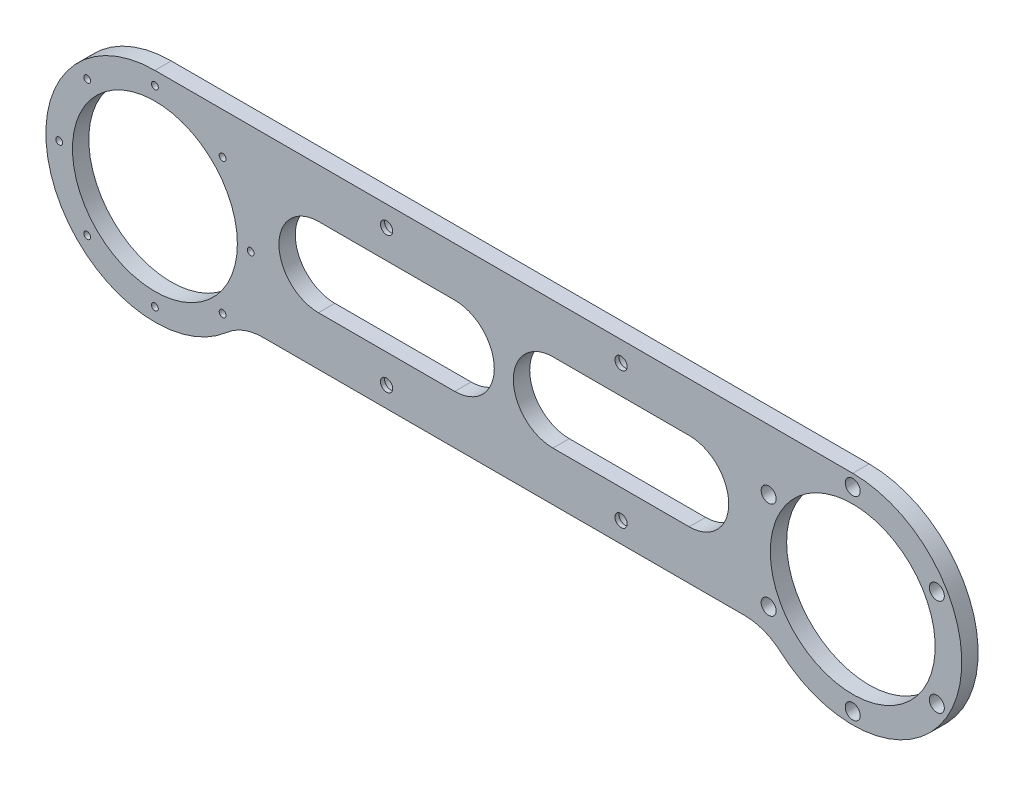
from build123d import *

# Parameters (mm, degrees)
SKETCH_1_R                   = 60.5
EXTRUDE_2_DEPTH              = 12
SKETCH_3_R                   = 60.5
CUT_EXTRUDE_2_DEPTH          = 4
HOLE_WIZARD_M8_2_D           = 9
HOLE_WIZARD_M8_2_CBORE_D     = 15
HOLE_WIZARD_M8_2_CBORE_DEPTH = 9
SKETCH_11_R                  = 18
CUT_EXTRUDE_5_DEPTH          = 472.497806181
SKETCH_12_R                  = 2.5
CUT_EXTRUDE_6_DEPTH          = 472.497806181
SKETCH_13_R                  = 60.5
CUT_EXTRUDE_7_DEPTH          = 472.412962521
SKETCH_14_R                  = 5.5
CUT_EXTRUDE_8_DEPTH          = 472.497806181


with BuildPart() as part:
    # 草图1 → 凸台-拉伸2 (new body)
    with BuildSketch(Plane.XY):
        with BuildLine():
            Line((-128, 82.886556409), (384, 82.886556409))
            ThreePointArc((384, 82.886556409), (458.833147735, -25.397714839), (331.084973779, -57.113443591))
            ThreePointArc((331.084973779, -57.113443591), (318.769596292, -49.696869724), (304.627460668, -47.113443591))
            Line((304.627460668, -47.113443591), (-48.627460668, -47.113443591))
            ThreePointArc((-48.627460668, -47.113443591), (-62.769596292, -49.696869724), (-75.084973779, -57.113443591))
            ThreePointArc((-75.084973779, -57.113443591), (-202.833147735, -25.397714839), (-128, 82.886556409))
        make_face()
        with Locations((-128, 2.886556409)):
            Circle(SKETCH_1_R, mode=Mode.SUBTRACT)
        with BuildLine():
            Line((-8, 46.886556409), (92, 46.886556409))
            ThreePointArc((92, 46.886556409), (121, 17.886556409), (92, -11.113443591))
            Line((92, -11.113443591), (-8, -11.113443591))
            ThreePointArc((-8, -11.113443591), (-37, 17.886556409), (-8, 46.886556409))
        make_face(mode=Mode.SUBTRACT)
        with BuildLine():
            Line((164, 46.886556409), (264, 46.886556409))
            ThreePointArc((264, 46.886556409), (293, 17.886556409), (264, -11.113443591))
            Line((264, -11.113443591), (164, -11.113443591))
            ThreePointArc((164, -11.113443591), (135, 17.886556409), (164, 46.886556409))
        make_face(mode=Mode.SUBTRACT)
    extrude(amount=EXTRUDE_2_DEPTH)

    # 草图3 → 切除-拉伸2 (cut)
    with BuildSketch(Plane.XY):
        with Locations((384, 2.886556409)):
            Circle(SKETCH_3_R)
    extrude(amount=CUT_EXTRUDE_2_DEPTH, mode=Mode.SUBTRACT)

    # M8 六角圆柱头螺钉的柱形沉头孔2 (through all)
    with Locations(Plane(origin=(0, 0, 0), x_dir=(-1, 0, 0), z_dir=(0, 0, -1))):
        with Locations((-214, 67.886556409), (-214, -32.113443591), (-42, 67.886556409), (-42, -32.113443591)):
            CounterBoreHole(HOLE_WIZARD_M8_2_D / 2, HOLE_WIZARD_M8_2_CBORE_D / 2, HOLE_WIZARD_M8_2_CBORE_DEPTH)

    # 草图11 → 切除-拉伸5 (cut, through all)
    with BuildSketch(Plane.XY):
        with Locations((384, 2.886556409)):
            Circle(SKETCH_11_R)
    extrude(amount=CUT_EXTRUDE_5_DEPTH, mode=Mode.SUBTRACT)

    # 草图12 → 切除-拉伸6 (cut, through all)
    with BuildSketch(Plane.XY.offset(12)):
        with Locations((-78.325748622, 52.560807787)):
            Circle(SKETCH_12_R)
        with Locations((-128, 73.136556409)):
            Circle(SKETCH_12_R)
        with Locations((-57.75, 2.886556409)):
            Circle(SKETCH_12_R)
        with Locations((-78.325748622, -46.78769497)):
            Circle(SKETCH_12_R)
        with Locations((-128, -67.363443591)):
            Circle(SKETCH_12_R)
        with Locations((-177.674251378, -46.78769497)):
            Circle(SKETCH_12_R)
        with Locations((-198.25, 2.886556409)):
            Circle(SKETCH_12_R)
        with Locations((-177.674251378, 52.560807787)):
            Circle(SKETCH_12_R)
    extrude(amount=-CUT_EXTRUDE_6_DEPTH, mode=Mode.SUBTRACT)

    # 草图13 → 切除-拉伸7 (cut, through all)
    with BuildSketch(Plane(origin=(0, 0, 4), x_dir=(-1, 0, 0), z_dir=(0, 0, -1))):
        with Locations((-384, 2.886556409)):
            Circle(SKETCH_13_R)
    extrude(amount=-CUT_EXTRUDE_7_DEPTH, mode=Mode.SUBTRACT)

    # 草图14 → 切除-拉伸8 (cut, through all)
    with BuildSketch(Plane(origin=(0, 0, 0), x_dir=(-1, 0, 0), z_dir=(0, 0, -1))):
        with Locations((-384, 74.136556409)):
            Circle(SKETCH_14_R)
        with Locations((-322.29568998, 38.511556409)):
            Circle(SKETCH_14_R)
        with Locations((-322.29568998, -32.738443591)):
            Circle(SKETCH_14_R)
        with Locations((-384, -68.363443591)):
            Circle(SKETCH_14_R)
        with Locations((-445.70431002, -32.738443591)):
            Circle(SKETCH_14_R)
        with Locations((-445.70431002, 38.511556409)):
            Circle(SKETCH_14_R)
    extrude(amount=-CUT_EXTRUDE_8_DEPTH, mode=Mode.SUBTRACT)


solid = part.part
